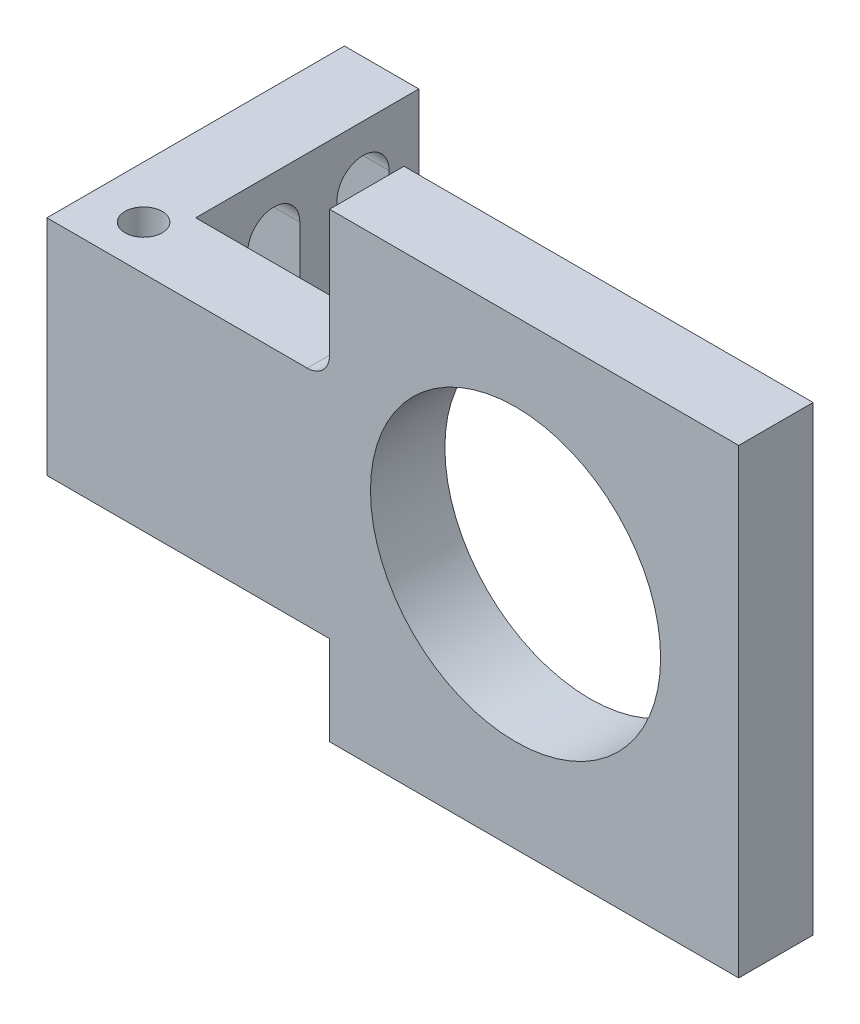
SolidWorks part; units mm, degrees
ref_plane "前视基准面" through (0, 0, 0) normal (0, 0, 1) x (1, 0, 0)
ref_plane "上视基准面" through (0, 0, 0) normal (0, 1, 0) x (1, 0, 0)
ref_plane "右视基准面" through (0, 0, 0) normal (1, 0, 0) x (0, 0, -1)
sketch "草图1" plane through (0, 0, 0) normal (0, 0, 1) x (1, 0, 0)
  line L0 (0, 0) -> (55, 0)
  line L1 (55, 0) -> (55, -50)
  line L2 (55, -50) -> (-38, -50)
  line L3 (-38, -50) -> (-38, -20)
  line L4 (-38, -20) -> (0, -20)
  line L5 (0, -20) -> (0, 0)
  dimension "D1" = 55
  dimension "D2" = 20
  dimension "D3" = 38
  dimension "D4" = 30
extrude "凸台-拉伸1" add sketch "草图1" along normal mid plane 10
fillet "圆角1" radius 3 1 edges at (0, -20, 0)
sketch "草图2" plane through (0, 0, -5) normal (0, 0, -1) x (-1, 0, 0)
  line L2 (-55, 0) -> (0, 0) construction
  line L3 (-55, -50) -> (-55, 0) construction
  circle A0 centre (-25, -30) radius 19.5
  dimension "D1" = 39
  dimension "D2" = 30
  dimension "D3" = 30
extrude "切除-拉伸1" cut sketch "草图2" against normal up to next
sketch "草图3" plane through (0, 0, -5) normal (0, 0, -1) x (-1, 0, 0)
  line L0 (-55, -27) -> (-44.2678, -27)
  line L1 (-55, -50) -> (-55, 0) construction
  line L2 (-44.2678, -27) -> (-44.2678, -33)
  line L3 (-44.2678, -33) -> (-55, -33)
  line L4 (-55, -33) -> (-55, -27)
  circle A0 centre (-25, -30) radius 19.5 construction
  dimension "D1" = 6
extrude "切除-拉伸2" [suppressed] cut sketch "草图3" against normal blind 6
sketch "草图4" plane through (0, 0, -5) normal (0, 0, -1) x (-1, 0, 0)
  line L0 (38, -50) -> (-55, -50) construction
  line L1 (38, -20) -> (28, -20)
  line L2 (38, -20) -> (38, -50)
  line L3 (38, -50) -> (28, -50)
  line L4 (28, -20) -> (28, -50)
  dimension "D1" = 10
extrude "凸台-拉伸2" add sketch "草图4" along normal blind 30
sketch "草图5" plane through (-28, 0, 0) normal (1, 0, 0) x (0, 0, -1)
  line L0 (27.5, -27.5) -> (27.5, -42.5) construction
  line L1 (31, -27.5) -> (31, -42.5)
  line L2 (24, -27.5) -> (24, -42.5)
  line L3 (15.5, -27.5) -> (15.5, -42.5) construction
  line L4 (19, -27.5) -> (19, -42.5)
  line L5 (12, -27.5) -> (12, -42.5)
  line L6 (35, -20) -> (35, -50) construction
  line L7 (27.5, -35) -> (35, -35) construction
  arc A0 (31, -27.5) -> (24, -27.5) centre (27.5, -27.5) ccw
  arc A1 (24, -42.5) -> (31, -42.5) centre (27.5, -42.5) ccw
  arc A2 (19, -27.5) -> (12, -27.5) centre (15.5, -27.5) ccw
  arc A3 (12, -42.5) -> (19, -42.5) centre (15.5, -42.5) ccw
  point P2 (27.5, -35)
  point P8 (15.5, -35)
  dimension "D1" = 3.5
  dimension "D2" = 4
  dimension "D3" = 5
  dimension "D4" = 15
extrude "切除-拉伸3" cut sketch "草图5" against normal up to next
hole_wizard "M6 螺纹孔1" positions "3D草图1" profile "草图6" tap size "M6" standard "GB"
sketch3d "3D草图1"
  line L3 (-3, -20, 5) -> (-38, -20, 5) construction
  line L4 (-38, -20, 5) -> (-38, -20, -35) construction
  point P0 (-31, -20, -1)
  dimension "D1" = 6
  dimension "D2" = 7
sketch "草图6" plane through (-31, -20, -1) normal (1, 0, 0) x (0, 0, 1)
  line L0 (0, 0) -> (0, 16.5022)
  line L1 (0, 16.5022) -> (2.5, 15)
  line L2 (2.5, 15) -> (2.5, 0)
  line L5 (2.5, 0) -> (0, 0)
  line L10 (0, 16.5022) -> (-2.5, 15) construction
  line L11 (0, -6.35) -> (0, 107.95) construction
  dimension "螺纹孔钻头直径" = 5
  dimension "螺纹孔钻头深度" = 15
  dimension "导头角度" = 118
cosmetic thread "孔螺蚊线1" parameters "D1"=12, "D2"=6
sketch "草图7" plane through (0, -50, 0) normal (0, -1, 0) x (1, 0, 0)
  line L0 (-28, -5) -> (55, -5) construction
  line L1 (55, 5) -> (0, 5)
  line L2 (55, 5) -> (55, -5)
  line L3 (55, -5) -> (0, -5)
  line L4 (0, 5) -> (0, -5)
  dimension "D1" = 55
extrude "凸台-拉伸3" add sketch "草图7" along normal blind 12
